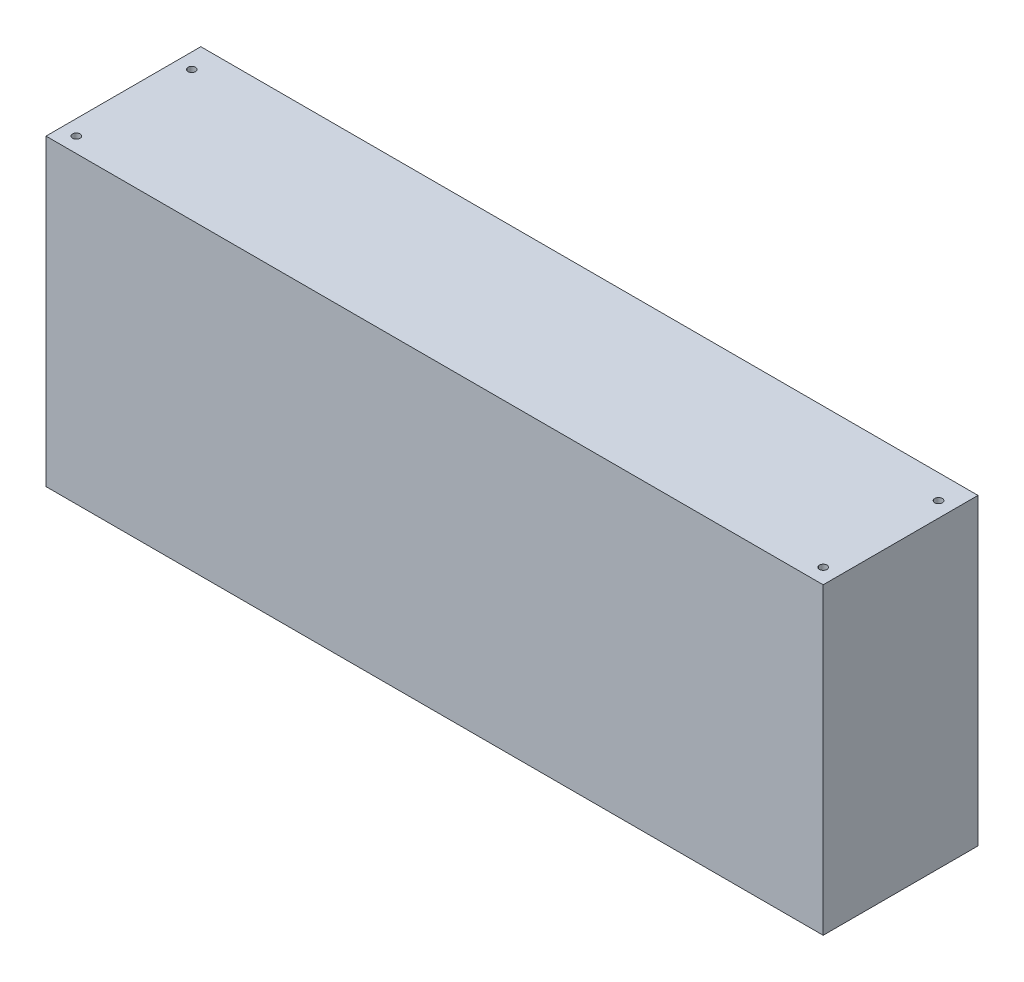
from build123d import *

# Parameters (mm, degrees)
SKETCH_1_W             = 256
SKETCH_1_H             = 100
EXTRUDE_1_DEPTH        = 25.5
HOLE_WIZARD_M3_1_D     = 2.5
HOLE_WIZARD_M3_1_DEPTH = 7.5
HOLE_WIZARD_M3_1_TIP   = 0.751075774


with BuildPart() as part:
    # 草图1 → 凸台-拉伸1 (new, symmetric)
    with BuildSketch(Plane.XY):
        Rectangle(SKETCH_1_W, SKETCH_1_H)
    extrude(amount=EXTRUDE_1_DEPTH, both=True)

    # M3 螺纹孔1
    with Locations(Plane(origin=(0, 50, 0), x_dir=(1, 0, 0), z_dir=(0, 1, 0))):
        with Locations((-123, 17.5), (-123, -20.5), (123, 17.5), (123, -20.5)):
            Hole(HOLE_WIZARD_M3_1_D / 2, depth=HOLE_WIZARD_M3_1_DEPTH)
            with Locations((0, 0, -(HOLE_WIZARD_M3_1_DEPTH + HOLE_WIZARD_M3_1_TIP / 2))):  # 118° drill point
                Cone(0, HOLE_WIZARD_M3_1_D / 2, HOLE_WIZARD_M3_1_TIP, mode=Mode.SUBTRACT)


solid = part.part
